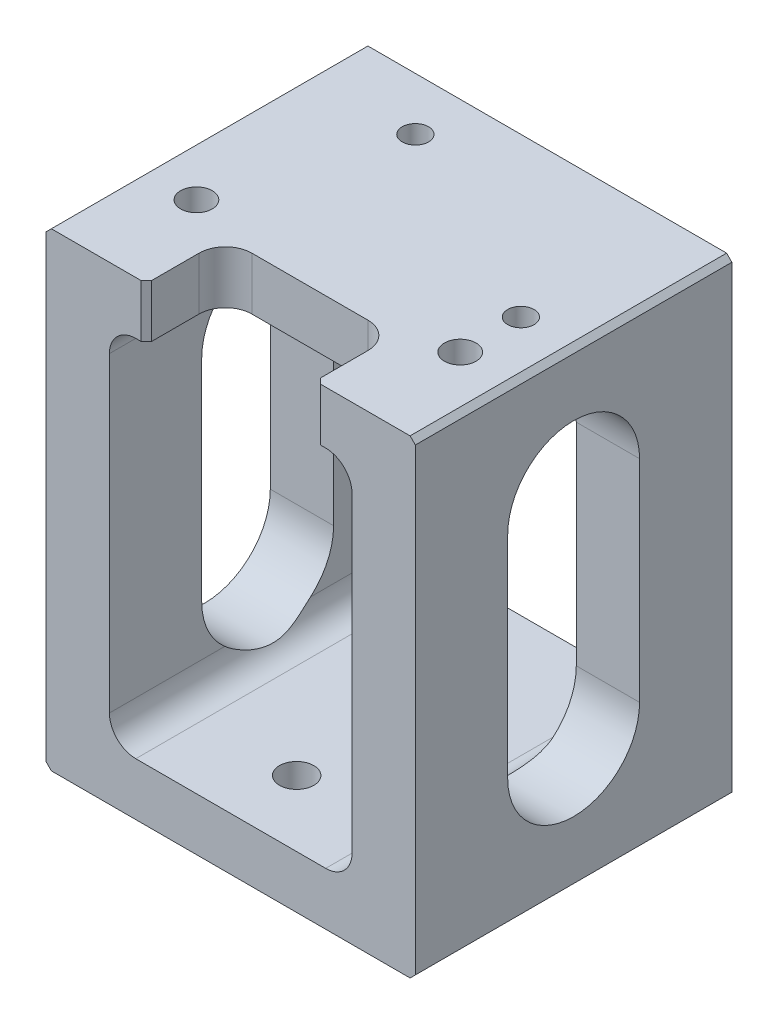
from build123d import *

# Parameters (mm, degrees)
SKETCH1_W                      = 70
SKETCH1_H                      = 89
SKETCH1_W_2                    = 46
SKETCH1_H_2                    = 69
BOSS_EXTRUDE1_DEPTH            = 30
FILLET2_R                      = 5
CUT_EXTRUDE1_DEPTH             = 118.136672311
M6_TAPPED_HOLE1_D              = 5
M6_TAPPED_HOLE1_DEPTH          = 15
M6_TAPPED_HOLE1_TIP            = 1.502151548
F_6_0_6_DIAMETER_HOLE1_D       = 6
F_6_0_6_DIAMETER_HOLE1_DEPTH   = 10
F_6_0_6_DIAMETER_HOLE1_TIP     = 1.802581857
F_6_5_6_5_DIAMETER_HOLE2_D     = 6.5
F_6_5_6_5_DIAMETER_HOLE2_DEPTH = 12
F_6_5_6_5_DIAMETER_HOLE2_TIP   = 1.952797012
CUT_EXTRUDE2_REACH             = 119.137
SKETCH10_W                     = 32
SKETCH10_H                     = 15
FILLET1_R                      = 5
CHAMFER1_SIZE                  = 1


with BuildPart() as part:
    # Sketch1 → Boss-Extrude1 (new, symmetric)
    with BuildSketch(Plane.XY):
        with Locations((35, 44.5)):
            Rectangle(SKETCH1_W, SKETCH1_H)
        with Locations((35, 44.5)):
            Rectangle(SKETCH1_W_2, SKETCH1_H_2, mode=Mode.SUBTRACT)
    extrude(amount=BOSS_EXTRUDE1_DEPTH, both=True)

    # Fillet2
    fillet2_edges = [part.edges().sort_by_distance(p)[0] for p in [
        (58, 10, 0),
        (58, 79, 0),
        (12, 79, 0),
        (12, 10, 0),
    ]]
    fillet(fillet2_edges, radius=FILLET2_R)

    # Sketch2 → Cut-Extrude1 (cut, through all)
    with BuildSketch(Plane.ZY):
        with BuildLine():
            Line((-12.5, 24.5), (-12.5, 64.5))
            ThreePointArc((-12.5, 64.5), (0, 77), (12.5, 64.5))
            Line((12.5, 64.5), (12.5, 24.5))
            ThreePointArc((12.5, 24.5), (0, 12), (-12.5, 24.5))
        make_face()
    extrude(amount=-CUT_EXTRUDE1_DEPTH, mode=Mode.SUBTRACT)

    # M6 Tapped Hole1
    with Locations(Plane(origin=(0, 89, 0), x_dir=(1, 0, 0), z_dir=(0, 1, 0))):
        with Locations((60, 0), (20, 20)):
            Hole(M6_TAPPED_HOLE1_D / 2, depth=M6_TAPPED_HOLE1_DEPTH)
            with Locations((0, 0, -(M6_TAPPED_HOLE1_DEPTH + M6_TAPPED_HOLE1_TIP / 2))):  # 118° drill point
                Cone(0, M6_TAPPED_HOLE1_D / 2, M6_TAPPED_HOLE1_TIP, mode=Mode.SUBTRACT)

    # Ø6.0 (6) Diameter Hole1
    with Locations(Plane(origin=(0, 89, 0), x_dir=(1, 0, 0), z_dir=(0, 1, 0))):
        with Locations((10, -11.5), (60, -11.5)):
            Hole(F_6_0_6_DIAMETER_HOLE1_D / 2, depth=F_6_0_6_DIAMETER_HOLE1_DEPTH)
            with Locations((0, 0, -(F_6_0_6_DIAMETER_HOLE1_DEPTH + F_6_0_6_DIAMETER_HOLE1_TIP / 2))):  # 118° drill point
                Cone(0, F_6_0_6_DIAMETER_HOLE1_D / 2, F_6_0_6_DIAMETER_HOLE1_TIP, mode=Mode.SUBTRACT)

    # Ø6.5 (6.5) Diameter Hole2
    with Locations(Plane(origin=(0, 0, 0), x_dir=(-1, 0, 0), z_dir=(0, -1, 0))):
        with Locations((-35, -17.5), (-35, 17.5)):
            Hole(F_6_5_6_5_DIAMETER_HOLE2_D / 2, depth=F_6_5_6_5_DIAMETER_HOLE2_DEPTH)
            with Locations((0, 0, -(F_6_5_6_5_DIAMETER_HOLE2_DEPTH + F_6_5_6_5_DIAMETER_HOLE2_TIP / 2))):  # 118° drill point
                Cone(0, F_6_5_6_5_DIAMETER_HOLE2_D / 2, F_6_5_6_5_DIAMETER_HOLE2_TIP, mode=Mode.SUBTRACT)

    # Sketch10 → Cut-Extrude2 (cut, up to next)
    with BuildSketch(Plane(origin=(0, 89, 0), x_dir=(1, 0, 0), z_dir=(0, 1, 0)), mode=Mode.PRIVATE) as cut_extrude2_sk1:
        with Locations((35, -22.5)):
            Rectangle(SKETCH10_W, SKETCH10_H)
    cut_extrude2_tool1 = extrude(cut_extrude2_sk1.sketch, amount=-CUT_EXTRUDE2_REACH, mode=Mode.PRIVATE) & part.part
    add(cut_extrude2_tool1.solids().sort_by_distance((35, 89, 22.5))[0], mode=Mode.SUBTRACT)

    # Fillet1
    fillet1_edges = [part.edges().sort_by_distance(p)[0] for p in [
        (51, 84, 15),
        (19, 84, 15),
    ]]
    fillet(fillet1_edges, radius=FILLET1_R)

    # Chamfer1
    chamfer1_edges = [part.edges().sort_by_distance(p)[0] for p in [
        (19, 84, 30),
        (51, 84, 30),
        (0, 89, 0),
        (70, 89, 0),
        (70, 0, 0),
        (0, 0, 0),
    ]]
    chamfer(chamfer1_edges, length=CHAMFER1_SIZE)


solid = part.part
